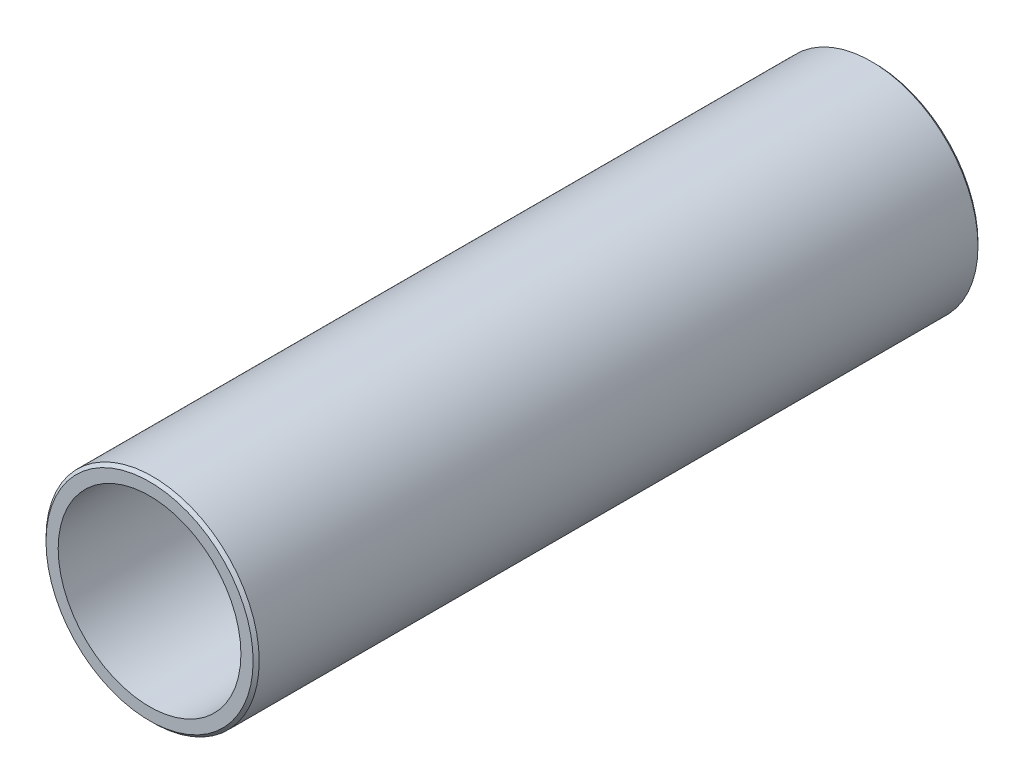
SolidWorks part; units mm, degrees
material "Q235B"
ref_plane "Front Plane" through (0, 0, 0) normal (0, 0, 1) x (1, 0, 0)
ref_plane "Top Plane" through (0, 0, 0) normal (0, 1, 0) x (1, 0, 0)
ref_plane "Right Plane" through (0, 0, 0) normal (1, 0, 0) x (0, 0, -1)
sketch "Sketch1" plane through (0, 0, 0) normal (0, 0, 1) x (1, 0, 0)
  circle A0 centre (0, 0) radius 35
  circle A1 centre (0, 0) radius 30
  dimension "D1" = 70
  dimension "D2" = 60
extrude "Boss-Extrude1" add sketch "Sketch1" along normal blind 238
chamfer "Chamfer1" distance 1 angle 45 2 edges at (35, 0, 0) (35, 0, 238)
